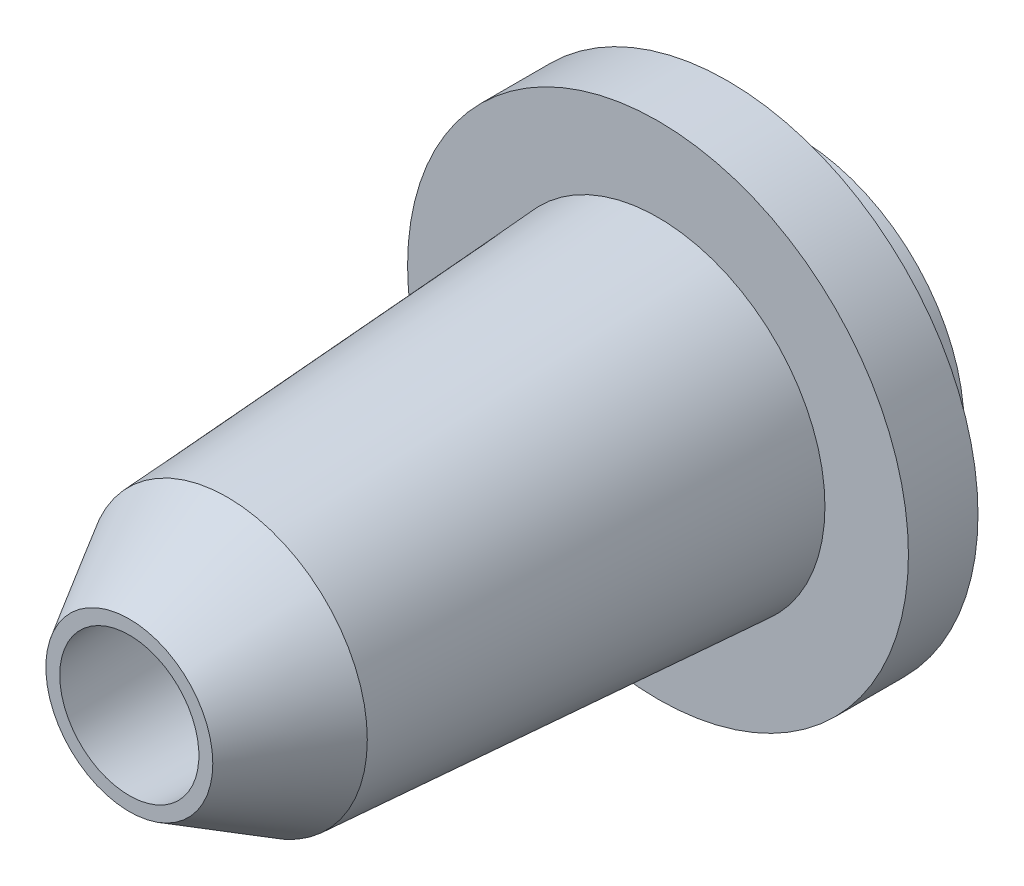
from build123d import *

# Parameters (mm, degrees)
SKETCH1_R           = 12
BOSS_EXTRUDE1_DEPTH = 5
SKETCH2_R           = 18
BOSS_EXTRUDE2_DEPTH = 5


with BuildPart() as part:
    # Sketch1 → Boss-Extrude1 (new body)
    with BuildSketch(Plane.XY):
        Circle(SKETCH1_R)
    extrude(amount=BOSS_EXTRUDE1_DEPTH)

    # Sketch2 → Boss-Extrude2 (add)
    with BuildSketch(Plane.XY.offset(5)):
        Circle(SKETCH2_R)
    extrude(amount=BOSS_EXTRUDE2_DEPTH)

    # Sketch3 → Revolve1 (revolve)
    with BuildSketch(Plane(origin=(0, 0, 0), x_dir=(0, 0, -1), z_dir=(1, 0, 0)), mode=Mode.PRIVATE) as revolve1_sk:
        Polygon((-10, 0), (-10, 12), (-40.959117986, 10.065055126), (-48, 6), (-48, 0), align=None)
    revolve(revolve1_sk.sketch.rotate(Axis((0, 0, 48), (0, 0, -1)), 90), axis=Axis((0, 0, 48), (0, 0, -1)))

    # Sketch5 → Cut-Revolve1 (revolve, cut)
    with BuildSketch(Plane(origin=(0, 0, 0), x_dir=(1, 0, 0), z_dir=(0, 1, 0)), mode=Mode.PRIVATE) as cut_revolve1_sk:
        Polygon((0, -48), (5, -48), (8, 0), (0, 0), align=None)
    revolve(cut_revolve1_sk.sketch.rotate(Axis((0, 0, 0), (0, 0, 1)), 180), axis=Axis((0, 0, 0), (0, 0, 1)), mode=Mode.SUBTRACT)


solid = part.part
